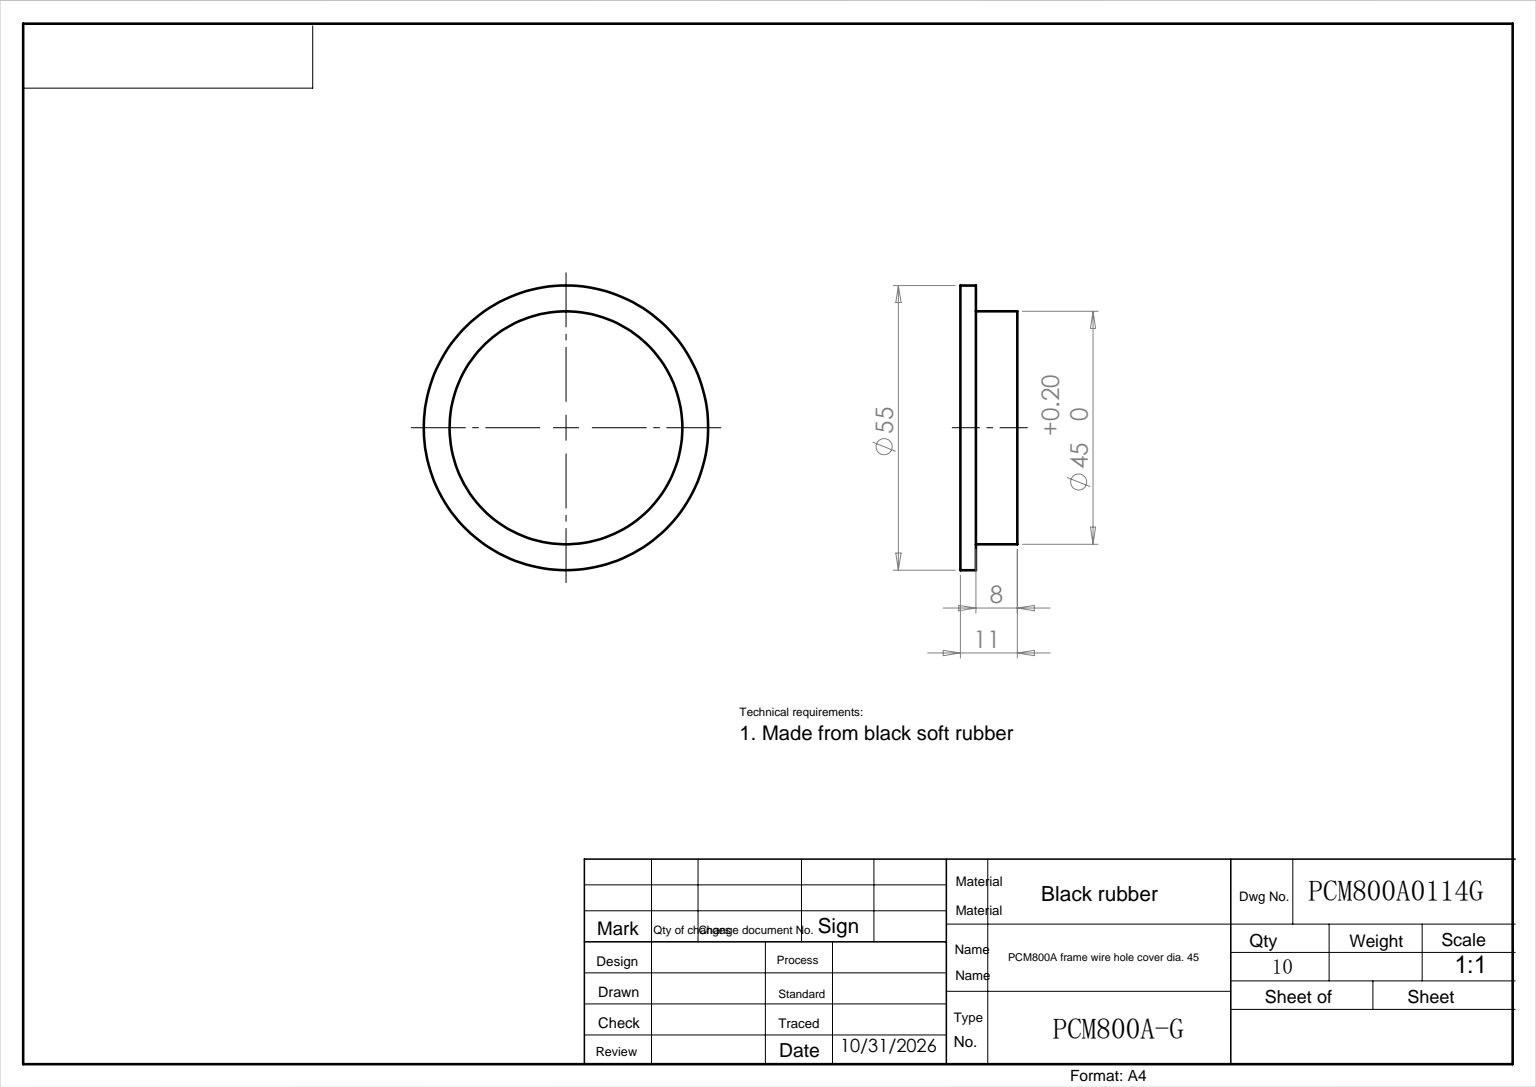
from build123d import *
from build123d.topology import SkipClean

# Parameters (mm, degrees)
REVOLVE_1_ANGLE           = 180
REVOLVE_1_OTHER_WAY_ANGLE = 180


with BuildPart() as part:
    # 草图1 → 旋转1 (revolve)
    with BuildSketch(Plane.XY):
        Polygon((0, 0), (-27.5, 0), (-27.5, 3), (-22.5, 3), (-22.5, 11), (0, 11), align=None)
    revolve(axis=Axis((0, 0, 0), (0, 1, 0)), revolution_arc=REVOLVE_1_ANGLE)

    # 草图1 → 旋转1 other way (revolve)
    with SkipClean():  # the faces are left unmerged after this step: merging them gives an invalid solid
        with BuildSketch(Plane.XY):
            Polygon((0, 0), (-27.5, 0), (-27.5, 3), (-22.5, 3), (-22.5, 11), (0, 11), align=None)
        revolve(axis=Axis((0, 0, 0), (0, -1, 0)), revolution_arc=REVOLVE_1_OTHER_WAY_ANGLE)


solid = part.part
